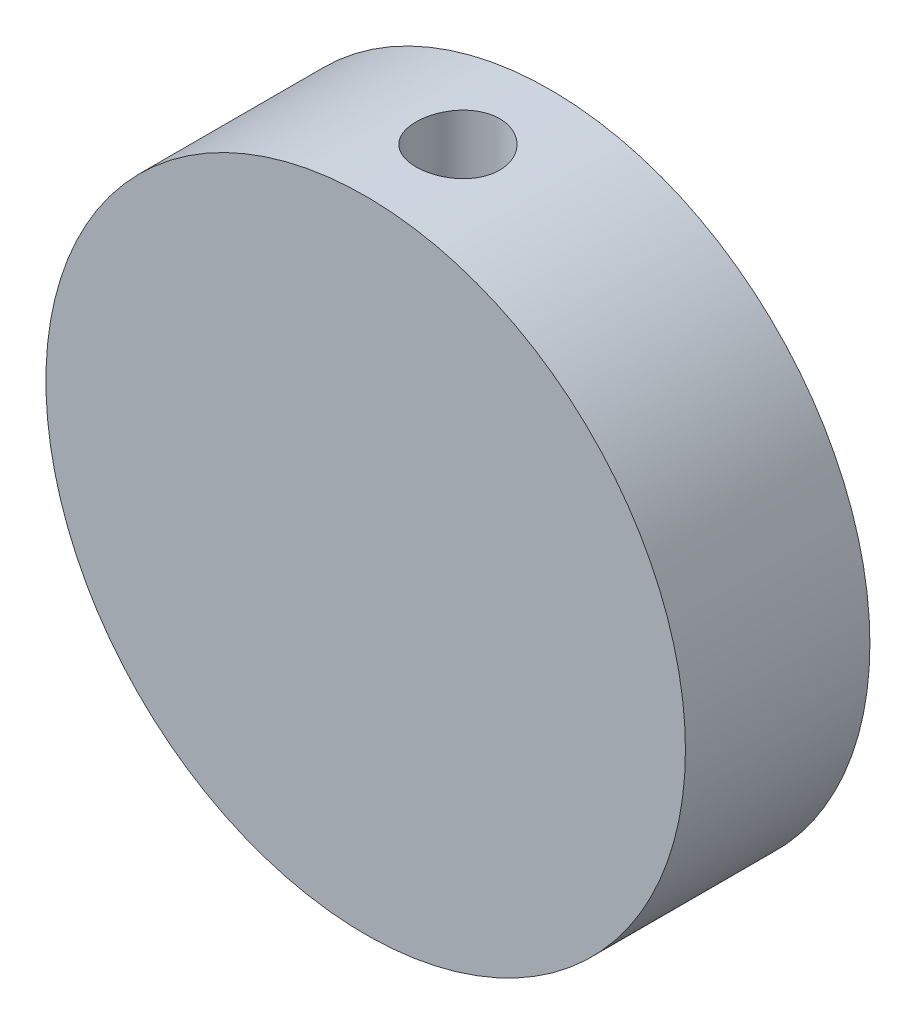
SolidWorks part; units mm, degrees
ref_plane "Front Plane" through (0, 0, 0) normal (0, 0, 1) x (1, 0, 0)
ref_plane "Top Plane" through (0, 0, 0) normal (0, 1, 0) x (1, 0, 0)
ref_plane "Right Plane" through (0, 0, 0) normal (1, 0, 0) x (0, 0, -1)
sketch "Sketch1" plane through (0, 0, 0) normal (0, 0, 1) x (1, 0, 0)
  line L0 (-106.5, 71.3) -> (-100, 71.3) construction
  line L1 (-68, 45.3) -> (-112, 45.3) construction
  circle A0 centre (-106.5, 71.3) radius 26
  dimension "D1" = 6.5
extrude "Boss-Extrude1" add sketch "Sketch1" along normal mid plane 15
sketch "Sketch2" plane through (0, 0, 0) normal (0, 0, 1) x (1, 0, 0)
  line L0 (-106.5, 71.3) -> (-106.5, 125.5934) construction
  line L1 (-132.5, 71.3) -> (-106.5, 71.3) construction
  line L2 (-106.5, 97.3) -> (-103.1, 97.3)
  line L3 (-103.1, 97.3) -> (-103.1, 87.263)
  line L4 (-103.1, 87.263) -> (-106.5, 85.3)
  line L5 (-106.5, 85.3) -> (-106.5, 97.3)
  circle A0 centre (-106.5, 71.3) radius 26 construction
  dimension "D1" = 90
  dimension "D2" = 60
  dimension "D3" = 6.8
  dimension "D4" = 12
revolve "Cut-Revolve1" cut sketch "Sketch2" angle 360 about L0
